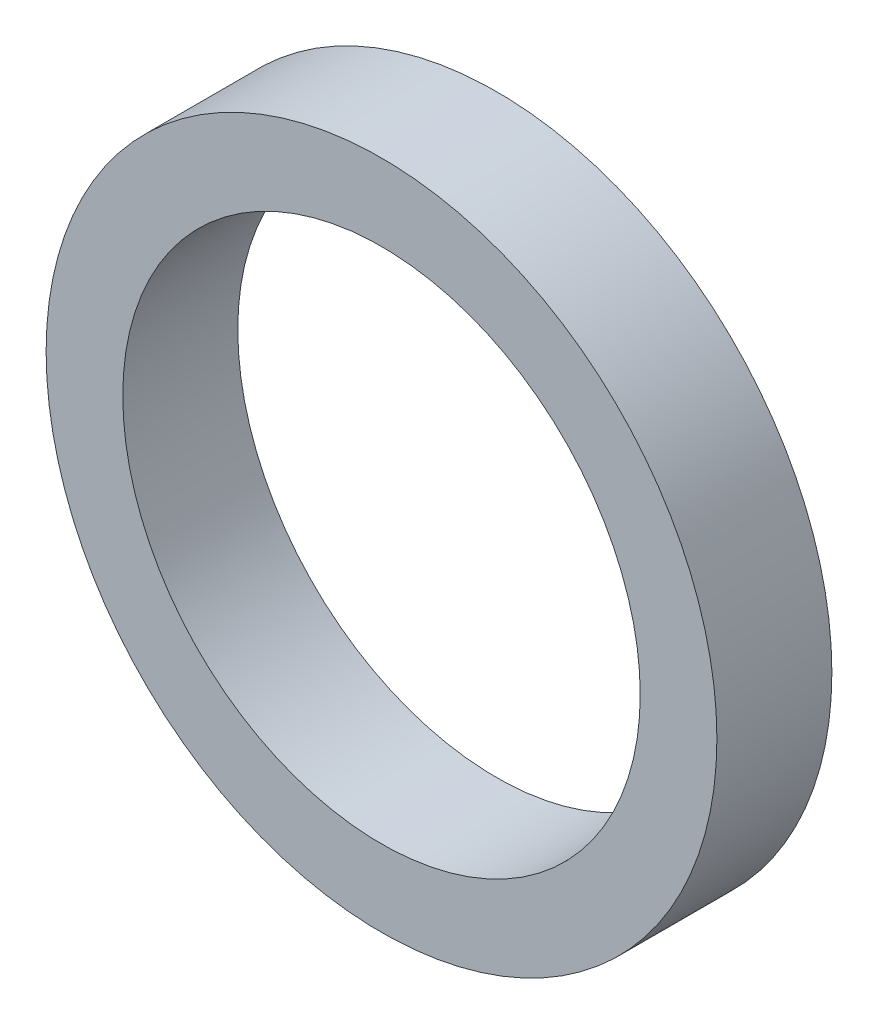
from build123d import *

# Parameters (mm, degrees)
SKETCH1_R           = 17.5
SKETCH1_R_2         = 13.5
BOSS_EXTRUDE1_DEPTH = 6


with BuildPart() as part:
    # Sketch1 → Boss-Extrude1 (new body)
    with BuildSketch(Plane.XY):
        Circle(SKETCH1_R)
        Circle(SKETCH1_R_2, mode=Mode.SUBTRACT)
    extrude(amount=BOSS_EXTRUDE1_DEPTH)


solid = part.part
